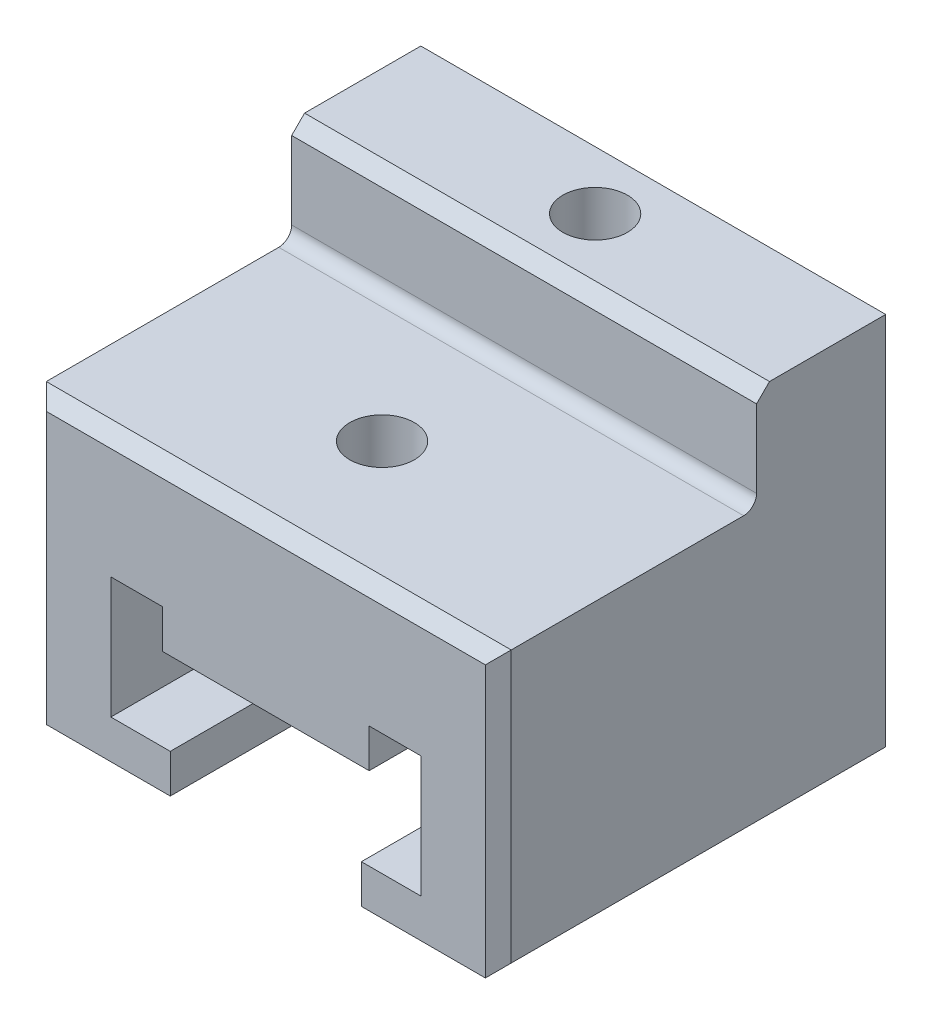
SolidWorks part; units mm, degrees
ref_plane "Front Plane" through (0, 0, 0) normal (0, 0, 1) x (1, 0, 0)
ref_plane "Top Plane" through (0, 0, 0) normal (0, 1, 0) x (1, 0, 0)
ref_plane "Right Plane" through (0, 0, 0) normal (1, 0, 0) x (0, 0, -1)
other "Configuration Table"
sketch "Sketch1" plane through (0, 0, 0) normal (0, 0, 1) x (1, 0, 0)
  line L0 (-3.7, -3.2) -> (-3.7, -4.7)
  line L1 (-3.7, -8.3) -> (-3.7, -3.2) construction
  line L2 (-3.7, -4.7) -> (-9, -4.7)
  line L3 (-9, -4.7) -> (-9, 10.3)
  line L4 (-9, 10.3) -> (9, 10.3)
  line L5 (0, 0) -> (0, 12.7218) construction
  line L7 (9, -4.7) -> (9, 10.3)
  line L8 (3.7, -4.7) -> (9, -4.7)
  line L9 (3.7, -3.2) -> (3.7, -4.7)
  line L10 (-3.7, -3.2) -> (-6, -3.2)
  line L11 (-6, -3) -> (-6, 1.3) construction
  line L12 (-3.7, -3.2) -> (-5.8, -3.2) construction
  line L13 (-6, -3.2) -> (-6, 1.5)
  line L14 (-6, 1.5) -> (-4, 1.5)
  line L15 (-4, 1.5) -> (-4, 0)
  line L16 (-4, 1.3) -> (-4, 0) construction
  line L17 (-4, 0) -> (0, 0)
  line L18 (0, 0) -> (4, 0)
  line L19 (-4, 0) -> (4, 0) construction
  line L20 (4, 0) -> (4, 1.5)
  line L21 (4, 1.5) -> (6, 1.5)
  line L22 (6, 1.5) -> (6, -3.2)
  line L23 (6, -3.2) -> (3.7, -3.2)
  point P14 (0, 10.3)
  dimension "D1" = 18
  dimension "D2" = 15
  dimension "D3" = 1.5
  dimension "D4" = 4.7
  dimension "D5" = 2
  dimension "D6" = 2.3
extrude "Boss-Extrude1" add sketch "Sketch1" against normal blind 15.5 from offset 14 contours L7 L4 L3 L2 L0 L10 L13 L14 L15 L17 L18 L20 L21 L22 L23 L9 L8 offset against normal yes
sketch "Sketch2" plane through (9, 0, 0) normal (1, 0, 0) x (0, 0, -1)
  line L0 (14, 6.3) -> (24, 6.3)
  line L1 (14, -4.7) -> (14, 10.3) construction
  line L2 (24, 6.3) -> (24, 10.3)
  line L3 (29.5, 10.3) -> (14, 10.3) construction
  line L4 (14, 6.3) -> (14, 10.3)
  line L5 (14, 10.3) -> (24, 10.3)
  dimension "D1" = 10
  dimension "D2" = 4
extrude "Cut-Extrude1" cut sketch "Sketch2" against normal through all
hole_wizard "M3 Tapped Hole1" positions "Sketch3" profile "Sketch4" tap size "M3" standard "GB"
sketch "Sketch3" plane through (0, 6.3, 0) normal (0, 1, 0) x (1, 0, 0)
  point P0 (-0.5, 19)
sketch "Sketch4" plane through (-0.5, 6.3, -19) normal (1, 0, 0) x (0, 0, 1)
  line L0 (0, 0) -> (0, 9.2511)
  line L1 (0, 9.2511) -> (1.25, 8.5)
  line L2 (1.25, 8.5) -> (1.25, 0)
  line L5 (1.25, 0) -> (0, 0)
  line L10 (0, 9.2511) -> (-1.25, 8.5) construction
  line L11 (0, -6.35) -> (0, 107.95) construction
  dimension "螺纹孔钻头直径" = 2.5
  dimension "螺纹孔钻头深度" = 8.5
  dimension "导头角度" = 118
cosmetic thread "Cosmetic Thread1" parameters "D1"=6, "D2"=3
hole_wizard "M3 Tapped Hole2" positions "Sketch5" profile "Sketch6" tap size "M3" standard "GB" end condition through all
sketch "Sketch5" plane through (0, 10.3, 0) normal (0, 1, 0) x (1, 0, 0)
  line L0 (0, 29.5) -> (0, 26.75) construction
  line L1 (-9, 29.5) -> (9, 29.5) construction
  line L3 (9, 26.75) -> (0, 26.75) construction
  line L4 (9, 29.5) -> (9, 24) construction
  point P0 (0, 26.75)
cosmetic thread "Cosmetic Thread2" parameters "D2"=3
sketch "Sketch6" plane through (0, 10.3, -26.75) normal (1, 0, 0) x (0, 0, 1)
  line L0 (0, 0) -> (0, 15)
  line L1 (0, 15) -> (1.25, 15)
  line L2 (1.25, 15) -> (1.25, 0)
  line L5 (1.25, 0) -> (0, 0)
  line L11 (0, -6.35) -> (0, 107.95) construction
  dimension "通孔螺纹孔钻头直径" = 2.5
  dimension "通孔螺纹孔钻头深度" = 15
chamfer "Chamfer1" distance 0.5 angle 45 9 edges at (0, 10.3, -24) (0, 6.3, -14) (-9, 0.8, -14) (-9, -4.7, -21.75) (-9, 2.8, -29.5) (0, 10.3, -29.5) (9, 0.8, -14) (9, -4.7, -21.75) (9, 2.8, -29.5)
fillet "Fillet1" radius 0.5 1 edges at (0, 6.3, -24)
